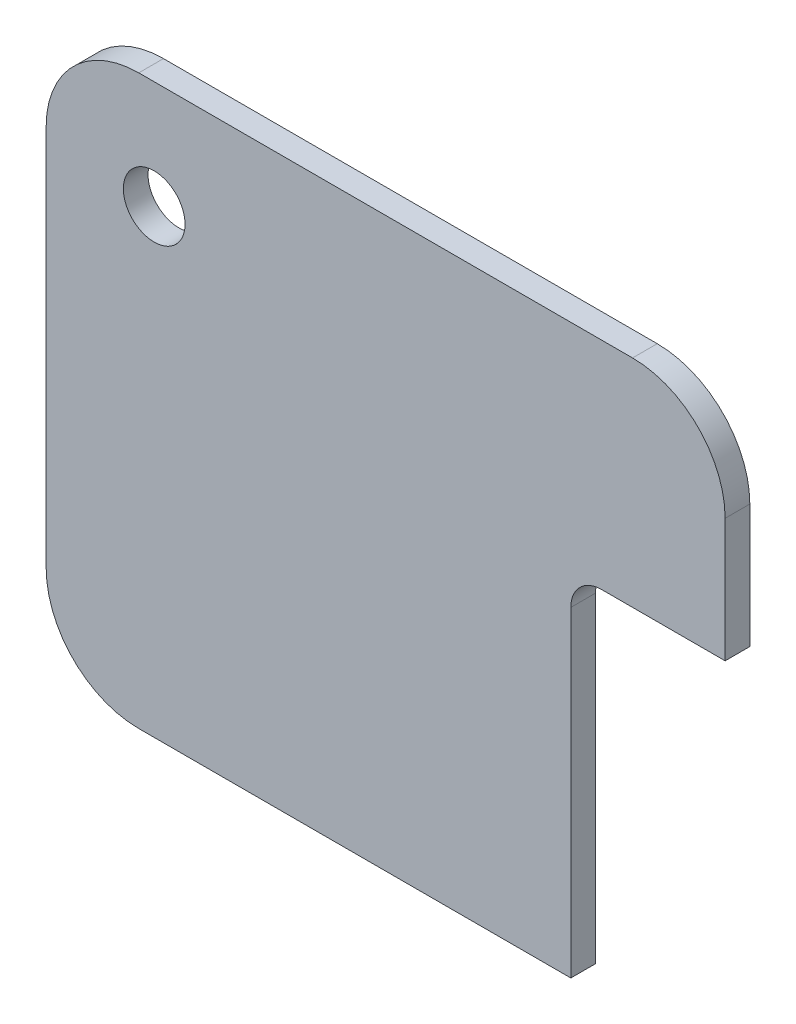
SolidWorks part; units mm, degrees
material "普通碳钢"
ref_plane "Front Plane" through (0, 0, 0) normal (0, 0, 1) x (1, 0, 0)
ref_plane "Top Plane" through (0, 0, 0) normal (0, 1, 0) x (1, 0, 0)
ref_plane "Right Plane" through (0, 0, 0) normal (1, 0, 0) x (0, 0, -1)
sketch "Sketch1" plane through (0, 0, 0) normal (0, 0, 1) x (1, 0, 0)
  line L0 (0, 30) -> (0, 154)
  line L1 (30, 184) -> (190, 184)
  line L2 (220, 154) -> (220, 114)
  line L3 (220, 114) -> (180, 114)
  line L4 (170, 104) -> (170, 0)
  line L5 (170, 0) -> (30, 0)
  arc A0 (190, 184) -> (220, 154) centre (190, 154) cw
  arc A1 (0, 30) -> (30, 0) centre (30, 30) ccw
  arc A2 (0, 154) -> (30, 184) centre (30, 154) cw
  arc A3 (180, 114) -> (170, 104) centre (180, 104) ccw
  circle A4 centre (35, 149) radius 10
  point P9 (220, 184)
  point P12 (0, 0)
  point P15 (0, 184)
  dimension "D5" = 30
  dimension "D6" = 10
  dimension "D9" = 20
  dimension "D1" = 220
  dimension "D2" = 70
  dimension "D3" = 184
  dimension "D4" = 170
  dimension "D7" = 35
  dimension "D8" = 35
extrude "Boss-Extrude1" add sketch "Sketch1" along normal blind 8
